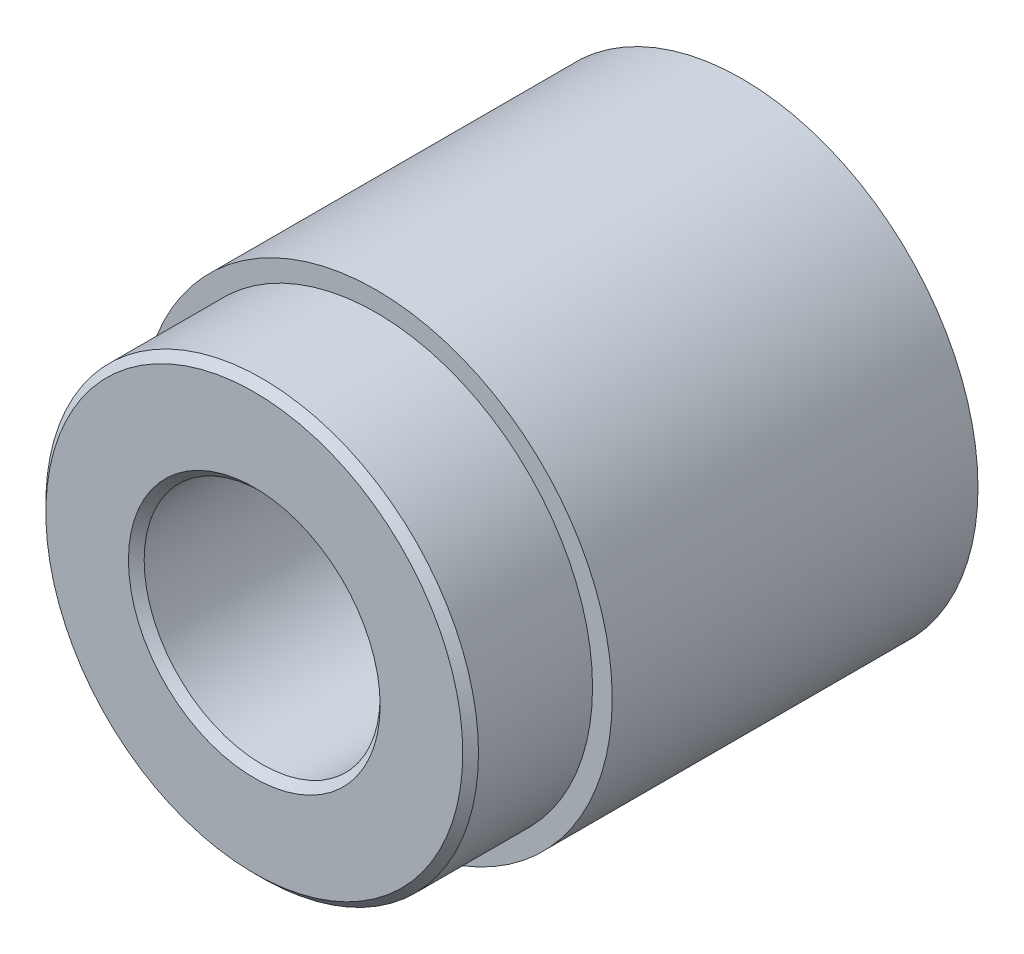
from build123d import *

# Parameters (mm, degrees)
SKETCH1_R           = 60
SKETCH1_R_2         = 30
BOSS_EXTRUDE1_DEPTH = 124
CUT_EXTRUDE1_START  = -31
SKETCH2_R           = 60
SKETCH2_R_2         = 55
CUT_EXTRUDE1_DEPTH  = 31
CHAMFER1_SIZE       = 2


with BuildPart() as part:
    # Sketch1 → Boss-Extrude1 (new body)
    with BuildSketch(Plane.XY):
        Circle(SKETCH1_R)
        Circle(SKETCH1_R_2, mode=Mode.SUBTRACT)
    extrude(amount=BOSS_EXTRUDE1_DEPTH)

    # Sketch2 → Cut-Extrude1 (cut)
    with BuildSketch(Plane.XY.offset(124).offset(CUT_EXTRUDE1_START)):
        Circle(SKETCH2_R)
        Circle(SKETCH2_R_2, mode=Mode.SUBTRACT)
    extrude(amount=CUT_EXTRUDE1_DEPTH, mode=Mode.SUBTRACT)

    # Chamfer1
    chamfer1_edges = [part.edges().sort_by_distance(p)[0] for p in [
        (-55, 0, 124),
        (-30, 0, 0),
        (-30, 0, 124),
    ]]
    chamfer(chamfer1_edges, length=CHAMFER1_SIZE)


solid = part.part
